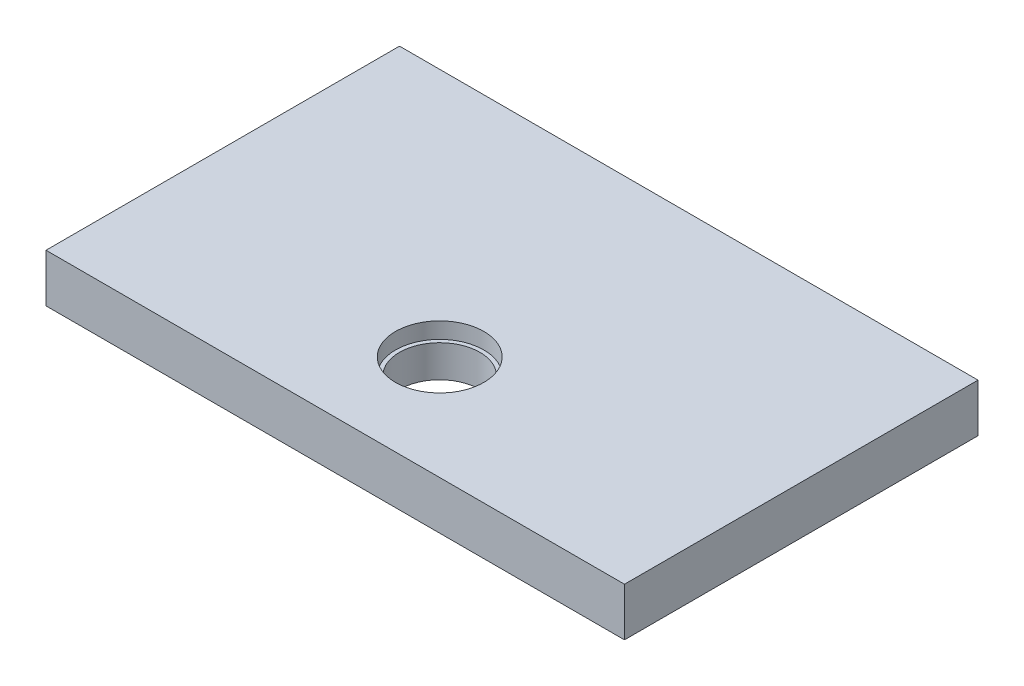
SolidWorks part; units mm, degrees
ref_plane "前视基准面" through (0, 0, 0) normal (0, 0, 1) x (1, 0, 0)
ref_plane "上视基准面" through (0, 0, 0) normal (0, 1, 0) x (1, 0, 0)
ref_plane "右视基准面" through (0, 0, 0) normal (1, 0, 0) x (0, 0, -1)
sketch "草图1" plane through (0, 0, 0) normal (0, 1, 0) x (1, 0, 0)
  line L1 (-180, -110) -> (180, -110)
  line L2 (-180, -110) -> (-180, 110)
  line L3 (-180, 110) -> (180, 110)
  line L4 (180, -110) -> (180, 110)
  line L5 (-180, -110) -> (180, 110) construction
  line L6 (-180, 110) -> (180, -110) construction
  point P0 (0, 0)
  dimension "D1" = 220
  dimension "D2" = 360
extrude "凸台-拉伸1" add sketch "草图1" along normal blind 30
sketch "草图2" plane through (0, 30, 0) normal (0, 1, 0) x (1, 0, 0)
  line L0 (180, -110) -> (180, 110) construction
  line L1 (180, 110) -> (-180, 110) construction
  circle A0 centre (0, -45) radius 27.5
  dimension "D1" = 55
  dimension "D2" = 180
  dimension "D3" = 155
extrude "切除-拉伸1" cut sketch "草图2" against normal blind 10
sketch "草图3" plane through (0, 30, 0) normal (0, 1, 0) x (1, 0, 0)
  line L0 (180, -110) -> (180, 110) construction
  line L1 (180, 110) -> (-180, 110) construction
  circle A0 centre (0, -45) radius 25
  dimension "D1" = 50
  dimension "D2" = 180
  dimension "D3" = 155
extrude "切除-拉伸2" cut sketch "草图3" against normal through all
